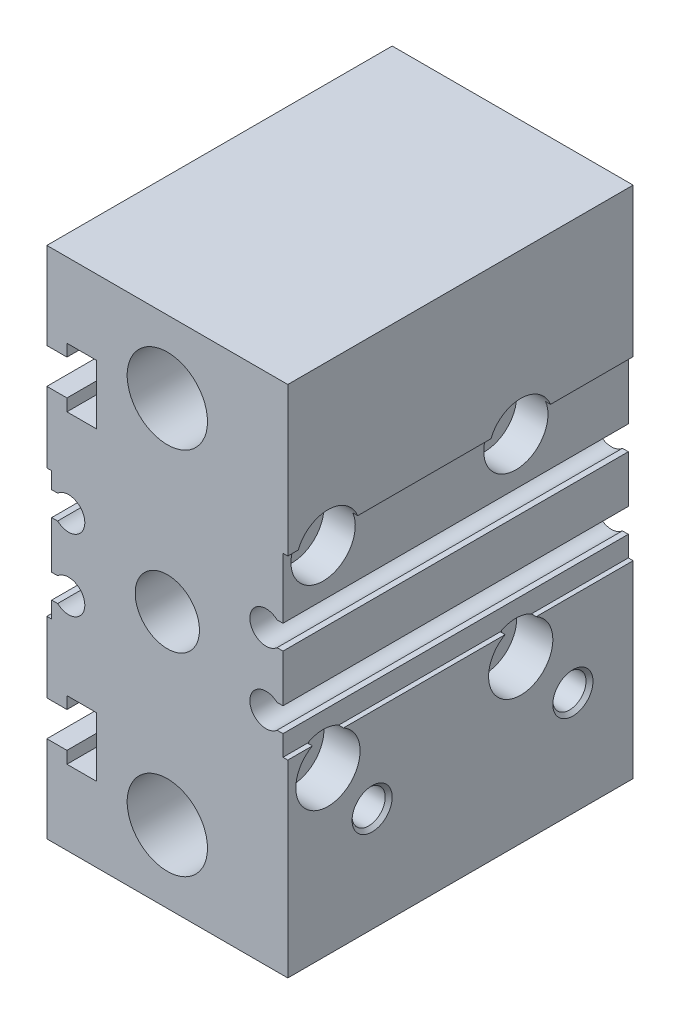
from build123d import *

# Parameters (mm, degrees)
BOSS_EXTRUDE1_DEPTH  = 43
HOLE1_D              = 4.134
HOLE1_DEPTH          = 5
HOLE1_CSINK_D        = 5
HOLE1_CSINK_ANGLE    = 90
HOLE1_TIP            = 1.193383006
HOLE2_D              = 4.134
HOLE2_DEPTH          = 5
HOLE2_CSINK_D        = 5
HOLE2_CSINK_ANGLE    = 90
HOLE2_TIP            = 1.193383006
HOLE3_D              = 4.134
HOLE3_DEPTH          = 5
HOLE3_CSINK_D        = 5
HOLE3_CSINK_ANGLE    = 90
HOLE3_TIP            = 1.193383006
HOLE4_D              = 4.134
HOLE4_DEPTH          = 5
HOLE4_CSINK_D        = 5
HOLE4_CSINK_ANGLE    = 90
HOLE4_TIP            = 1.193383006
HOLE5_D              = 3
HOLE5_DEPTH          = 6
HOLE5_TIP            = 0.866025404
CUT_EXTRUDE1_DEPTH   = 3
HOLE6_D              = 3
HOLE6_DEPTH          = 6
HOLE6_TIP            = 0.866025404
HOLE7_D              = 10
HOLE8_D              = 10
HOLE9_D              = 3
HOLE9_DEPTH          = 6
HOLE9_TIP            = 0.866025404
CUT_EXTRUDE2_DEPTH   = 3
HOLE10_D             = 3
HOLE10_DEPTH         = 6
HOLE10_TIP           = 0.866025404
LPATTERN1_COUNT      = 2
LPATTERN1_PITCH      = 22
LPATTERN1_COUNT_DIR2 = 2
LPATTERN1_PITCH_DIR2 = 56


with BuildPart() as part:
    # Sketch1 → Boss-Extrude1 (new body)
    with BuildSketch(Plane.XY):
        with BuildLine():
            Line((-15, 32), (-15, 21.2))
            Line((-15, 21.2), (-12.5, 21.2))
            Line((-12.5, 21.2), (-12.5, 22.7))
            Line((-12.5, 22.7), (-8.8, 22.7))
            Line((-8.8, 22.7), (-8.8, 15.3))
            Line((-8.8, 15.3), (-12.5, 15.3))
            Line((-12.5, 15.3), (-12.5, 16.8))
            Line((-12.5, 16.8), (-15, 16.8))
            Line((-15, 16.8), (-15, 8))
            Line((-15, 8), (-14.4, 8))
            Line((-14.4, 8), (-14.4, 5.95))
            Line((-14.4, 5.95), (-13.660376786, 5.95))
            ThreePointArc((-13.660376786, 5.95), (-10.275, 4.45), (-13.660376786, 2.95))
            Line((-13.660376786, 2.95), (-14.4, 2.95))
            Line((-14.4, 2.95), (-14.4, -2.95))
            Line((-14.4, -2.95), (-13.660376786, -2.95))
            ThreePointArc((-13.660376786, -2.95), (-10.275, -4.45), (-13.660376786, -5.95))
            Line((-13.660376786, -5.95), (-14.4, -5.95))
            Line((-14.4, -5.95), (-14.4, -8))
            Line((-14.4, -8), (-15, -8))
            Line((-15, -8), (-15, -16.8))
            Line((-15, -16.8), (-12.5, -16.8))
            Line((-12.5, -16.8), (-12.5, -15.3))
            Line((-12.5, -15.3), (-8.8, -15.3))
            Line((-8.8, -15.3), (-8.8, -22.7))
            Line((-8.8, -22.7), (-12.5, -22.7))
            Line((-12.5, -22.7), (-12.5, -21.2))
            Line((-12.5, -21.2), (-15, -21.2))
            Line((-15, -21.2), (-15, -32))
            Line((-15, -32), (15, -32))
            Line((15, -32), (15, -8.5))
            Line((15, -8.5), (14.4, -8.5))
            Line((14.4, -8.5), (14.4, -5.95))
            Line((14.4, -5.95), (13.660376786, -5.95))
            ThreePointArc((13.660376786, -5.95), (10.275, -4.45), (13.660376786, -2.95))
            Line((13.660376786, -2.95), (14.4, -2.95))
            Line((14.4, -2.95), (14.4, 2.95))
            Line((14.4, 2.95), (13.660376786, 2.95))
            ThreePointArc((13.660376786, 2.95), (10.275, 4.45), (13.660376786, 5.95))
            Line((13.660376786, 5.95), (14.4, 5.95))
            Line((14.4, 5.95), (14.4, 13.5))
            Line((14.4, 13.5), (15, 13.5))
            Line((15, 13.5), (15, 32))
            Line((15, 32), (-15, 32))
        make_face()
    extrude(amount=-BOSS_EXTRUDE1_DEPTH)

    # Sketch2 → Cut-Revolve1 (revolve, cut)
    with BuildSketch(Plane(origin=(0, 0, 0), x_dir=(0, 0, -1), z_dir=(1, 0, 0)), mode=Mode.PRIVATE) as cut_revolve1_sk:
        Polygon((0, 0), (0, 4), (10.5, 4), (10.5, 8), (25.5, 8), (25.5, 0), align=None)
    revolve(cut_revolve1_sk.sketch.rotate(Axis((0, 0, -25.5), (0, 0, 1)), 270), axis=Axis((0, 0, -25.5), (0, 0, 1)), mode=Mode.SUBTRACT)

    # Hole1
    with Locations(Plane(origin=(15, 0, 0), x_dir=(0, 0, -1), z_dir=(1, 0, 0))):
        with Locations((10.5, -19)):
            CounterSinkHole(HOLE1_D / 2, HOLE1_CSINK_D / 2, depth=HOLE1_DEPTH, counter_sink_angle=HOLE1_CSINK_ANGLE)
            with Locations((0, 0, -(HOLE1_DEPTH + HOLE1_TIP / 2))):  # 120° drill point
                Cone(0, HOLE1_D / 2, HOLE1_TIP, mode=Mode.SUBTRACT)

    # Hole2
    with Locations(Plane(origin=(15, 0, 0), x_dir=(0, 0, -1), z_dir=(1, 0, 0))):
        with Locations((35.5, -19)):
            CounterSinkHole(HOLE2_D / 2, HOLE2_CSINK_D / 2, depth=HOLE2_DEPTH, counter_sink_angle=HOLE2_CSINK_ANGLE)
            with Locations((0, 0, -(HOLE2_DEPTH + HOLE2_TIP / 2))):  # 120° drill point
                Cone(0, HOLE2_D / 2, HOLE2_TIP, mode=Mode.SUBTRACT)

    # Sketch7 → Cut-Revolve2 (revolve, cut)
    with BuildSketch(Plane(origin=(0, -12, 0), x_dir=(1, 0, 0), z_dir=(0, 1, 0)), mode=Mode.PRIVATE) as cut_revolve2_sk:
        Polygon((-15, 5), (-15, 7.5), (-14.567, 7.067), (-5, 7.067), (-5, 7.15), (10.5, 7.15), (10.5, 9), (15, 9), (15, 5), align=None)
    revolve(cut_revolve2_sk.sketch.rotate(Axis((15, -12, -5), (-1, 0, 0)), 180), axis=Axis((15, -12, -5), (-1, 0, 0)), mode=Mode.SUBTRACT)

    # Sketch8 → Cut-Revolve3 (revolve, cut)
    with BuildSketch(Plane(origin=(0, -12, 0), x_dir=(1, 0, 0), z_dir=(0, 1, 0)), mode=Mode.PRIVATE) as cut_revolve3_sk:
        Polygon((-15, 29), (-15, 31.5), (-14.567, 31.067), (-5, 31.067), (-5, 31.15), (10.5, 31.15), (10.5, 33), (15, 33), (15, 29), align=None)
    revolve(cut_revolve3_sk.sketch.rotate(Axis((15, -12, -29), (-1, 0, 0)), 180), axis=Axis((15, -12, -29), (-1, 0, 0)), mode=Mode.SUBTRACT)

    # Sketch9 → Cut-Revolve4 (revolve, cut)
    with BuildSketch(Plane(origin=(0, 12, 0), x_dir=(1, 0, 0), z_dir=(0, 1, 0)), mode=Mode.PRIVATE) as cut_revolve4_sk:
        Polygon((-15, 5), (-15, 7.5), (-14.567, 7.067), (-5, 7.067), (-5, 7.15), (10.5, 7.15), (10.5, 9), (15, 9), (15, 5), align=None)
    revolve(cut_revolve4_sk.sketch.rotate(Axis((15, 12, -5), (-1, 0, 0)), 180), axis=Axis((15, 12, -5), (-1, 0, 0)), mode=Mode.SUBTRACT)

    # Sketch10 → Cut-Revolve5 (revolve, cut)
    with BuildSketch(Plane(origin=(0, 12, 0), x_dir=(1, 0, 0), z_dir=(0, 1, 0)), mode=Mode.PRIVATE) as cut_revolve5_sk:
        Polygon((-15, 29), (-15, 31.5), (-14.567, 31.067), (-5, 31.067), (-5, 31.15), (10.5, 31.15), (10.5, 33), (15, 33), (15, 29), align=None)
    revolve(cut_revolve5_sk.sketch.rotate(Axis((15, 12, -29), (-1, 0, 0)), 180), axis=Axis((15, 12, -29), (-1, 0, 0)), mode=Mode.SUBTRACT)

    # Hole3
    with Locations(Plane(origin=(0, -32, 0), x_dir=(-1, 0, 0), z_dir=(0, -1, 0))):
        with Locations((-10, 10.5)):
            CounterSinkHole(HOLE3_D / 2, HOLE3_CSINK_D / 2, depth=HOLE3_DEPTH, counter_sink_angle=HOLE3_CSINK_ANGLE)
            with Locations((0, 0, -(HOLE3_DEPTH + HOLE3_TIP / 2))):  # 120° drill point
                Cone(0, HOLE3_D / 2, HOLE3_TIP, mode=Mode.SUBTRACT)

    # Hole4
    with Locations(Plane(origin=(0, -32, 0), x_dir=(-1, 0, 0), z_dir=(0, -1, 0))):
        with Locations((-10, 24.5)):
            CounterSinkHole(HOLE4_D / 2, HOLE4_CSINK_D / 2, depth=HOLE4_DEPTH, counter_sink_angle=HOLE4_CSINK_ANGLE)
            with Locations((0, 0, -(HOLE4_DEPTH + HOLE4_TIP / 2))):  # 120° drill point
                Cone(0, HOLE4_D / 2, HOLE4_TIP, mode=Mode.SUBTRACT)

    # Hole5
    with Locations(Plane.ZY.offset(15)):
        with Locations((-17, 12)):
            Hole(HOLE5_D / 2, depth=HOLE5_DEPTH)
            with Locations((0, 0, -(HOLE5_DEPTH + HOLE5_TIP / 2))):  # 120° drill point
                Cone(0, HOLE5_D / 2, HOLE5_TIP, mode=Mode.SUBTRACT)

    # Sketch17 → Cut-Extrude1 (cut)
    with BuildSketch(Plane(origin=(-15, 0, 0), x_dir=(0, 0, -1), z_dir=(1, 0, 0))):
        with BuildLine():
            Line((18.5, 11.75), (18.5, 12.25))
            ThreePointArc((18.5, 12.25), (17, 13.75), (15.5, 12.25))
            Line((15.5, 12.25), (15.5, 11.75))
            ThreePointArc((15.5, 11.75), (17, 10.25), (18.5, 11.75))
        make_face()
    extrude(amount=CUT_EXTRUDE1_DEPTH, mode=Mode.SUBTRACT)

    # Hole6
    with Locations(Plane.ZY.offset(15)):
        with Locations((-17, -12)):
            Hole(HOLE6_D / 2, depth=HOLE6_DEPTH)
            with Locations((0, 0, -(HOLE6_DEPTH + HOLE6_TIP / 2))):  # 120° drill point
                Cone(0, HOLE6_D / 2, HOLE6_TIP, mode=Mode.SUBTRACT)

    # Hole7 (through all)
    with Locations(Plane.XY):
        with Locations((0, 23)):
            Hole(HOLE7_D / 2)

    # Hole8 (through all)
    with Locations(Plane.XY):
        with Locations((0, -23)):
            Hole(HOLE8_D / 2)

    # Hole9
    with Locations(Plane(origin=(0, 0, -43), x_dir=(-1, 0, 0), z_dir=(0, 0, -1))):
        with Locations((0, 12)):
            Hole(HOLE9_D / 2, depth=HOLE9_DEPTH)
            with Locations((0, 0, -(HOLE9_DEPTH + HOLE9_TIP / 2))):  # 120° drill point
                Cone(0, HOLE9_D / 2, HOLE9_TIP, mode=Mode.SUBTRACT)

    # Sketch26 → Cut-Extrude2 (cut)
    with BuildSketch(Plane.XY.offset(-43)):
        with BuildLine():
            Line((1.5, 11.75), (1.5, 12.25))
            ThreePointArc((1.5, 12.25), (0, 13.75), (-1.5, 12.25))
            Line((-1.5, 12.25), (-1.5, 11.75))
            ThreePointArc((-1.5, 11.75), (0, 10.25), (1.5, 11.75))
        make_face()
    extrude(amount=CUT_EXTRUDE2_DEPTH, mode=Mode.SUBTRACT)

    # Hole10
    with Locations(Plane(origin=(0, 0, -43), x_dir=(-1, 0, 0), z_dir=(0, 0, -1))):
        with Locations((0, -12)):
            Hole(HOLE10_D / 2, depth=HOLE10_DEPTH)
            with Locations((0, 0, -(HOLE10_DEPTH + HOLE10_TIP / 2))):  # 120° drill point
                Cone(0, HOLE10_D / 2, HOLE10_TIP, mode=Mode.SUBTRACT)

    # Sketch29 → Hole11 (revolve, cut)
    with BuildSketch(Plane(origin=(11, 28, -43), x_dir=(0, 1, 0), z_dir=(1, 0, 0))):
        Polygon((0, 0), (0, 13.193383006), (2.067, 12), (2.067, 0.433), (2.5, 0), align=None)
    hole11 = revolve(axis=Axis((11, 28, -57.308894879), (0, 0, 1)), mode=Mode.SUBTRACT)

    # LPattern1: Hole11 2 × 2
    with Locations(*[(-i * LPATTERN1_PITCH, -j * LPATTERN1_PITCH_DIR2, 0) for i in range(LPATTERN1_COUNT) for j in range(LPATTERN1_COUNT_DIR2) if (i, j) != (0, 0)]):
        add(hole11, mode=Mode.SUBTRACT)


solid = part.part
